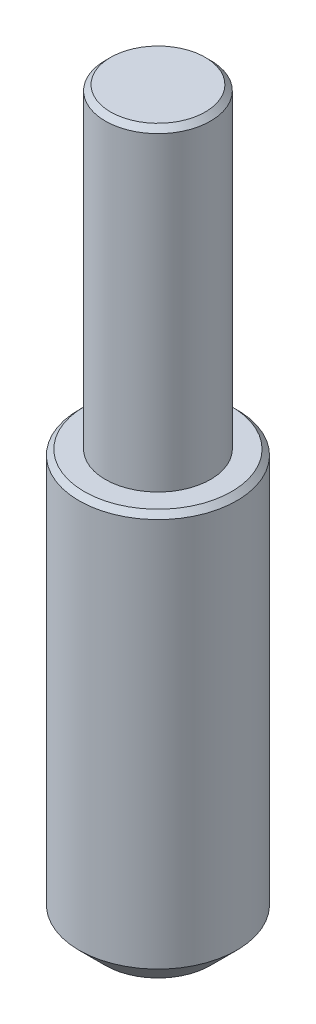
from build123d import *


with BuildPart() as part:
    # Sketch1 → Revolve1 (revolve)
    with BuildSketch(Plane.XY, mode=Mode.PRIVATE) as revolve1_sk:
        Polygon((0, 0), (-2, 0), (-3, 1), (-3, 15.8), (-2.8, 16), (-2, 16), (-2, 27.8), (-1.8, 28), (0, 28), align=None)
    revolve(revolve1_sk.sketch.rotate(Axis((0, 13.359319257, 0), (0, -1, 0)), 270), axis=Axis((0, 13.359319257, 0), (0, -1, 0)))


solid = part.part
